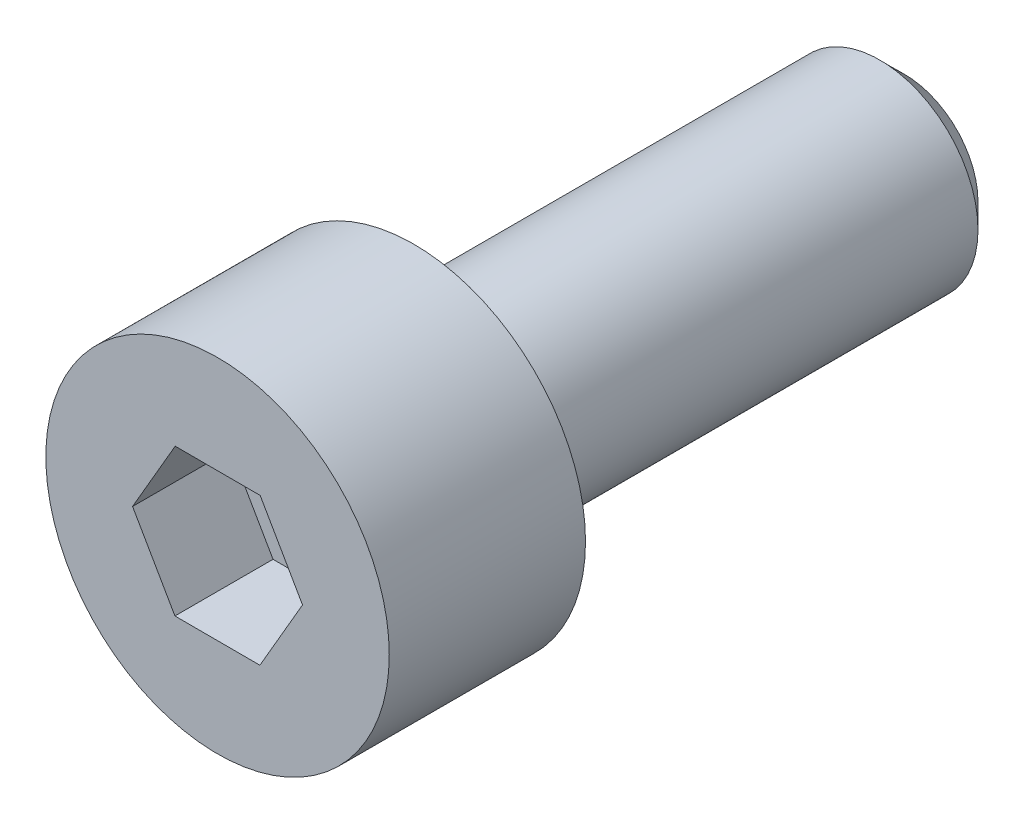
SolidWorks part; units mm, degrees
material "SUS304"
ref_plane "前视基准面" through (0, 0, 0) normal (0, 0, 1) x (1, 0, 0)
ref_plane "上视基准面" through (0, 0, 0) normal (0, 1, 0) x (1, 0, 0)
ref_plane "右视基准面" through (0, 0, 0) normal (1, 0, 0) x (0, 0, -1)
sketch "草图1" plane through (0, 0, 0) normal (0, 0, 1) x (1, 0, 0)
  circle A0 centre (0, 0) radius 2
  dimension "D1" = 4
extrude "凸台-拉伸1" add sketch "草图1" along normal blind 10
sketch "草图2" plane through (0, 0, 10) normal (0, 0, 1) x (1, 0, 0)
  circle A0 centre (0, 0) radius 3.5
  dimension "D1" = 7
extrude "凸台-拉伸2" add sketch "草图2" along normal blind 4
sketch "草图3" plane through (0, 0, 14) normal (0, 0, 1) x (1, 0, 0)
  line L0 (-0.8632, 1.5017) -> (-1.732, 0.0033)
  line L1 (0.8632, -1.5017) -> (1.732, -0.0033)
  line L2 (1.732, -0.0033) -> (0.8689, 1.4983)
  line L3 (0.8689, 1.4983) -> (-0.8632, 1.5017)
  line L4 (-1.732, 0.0033) -> (-0.8689, -1.4983)
  line L5 (-0.8689, -1.4983) -> (0.8632, -1.5017)
  circle A0 centre (0, 0) radius 1.5 construction
  dimension "D1" = 3
extrude "切除-拉伸1" cut sketch "草图3" against normal blind 2
chamfer "倒角1" distance 0.5 angle 45 1 edges at (2, 0, 0)
sketch "草图4" plane through (0, 0, 12) normal (0, 0, 1) x (1, 0, 0)
  circle A0 centre (0, 0) radius 0.75
  dimension "D1" = 1.5
extrude "切除-拉伸2" cut sketch "草图4" against normal through all
